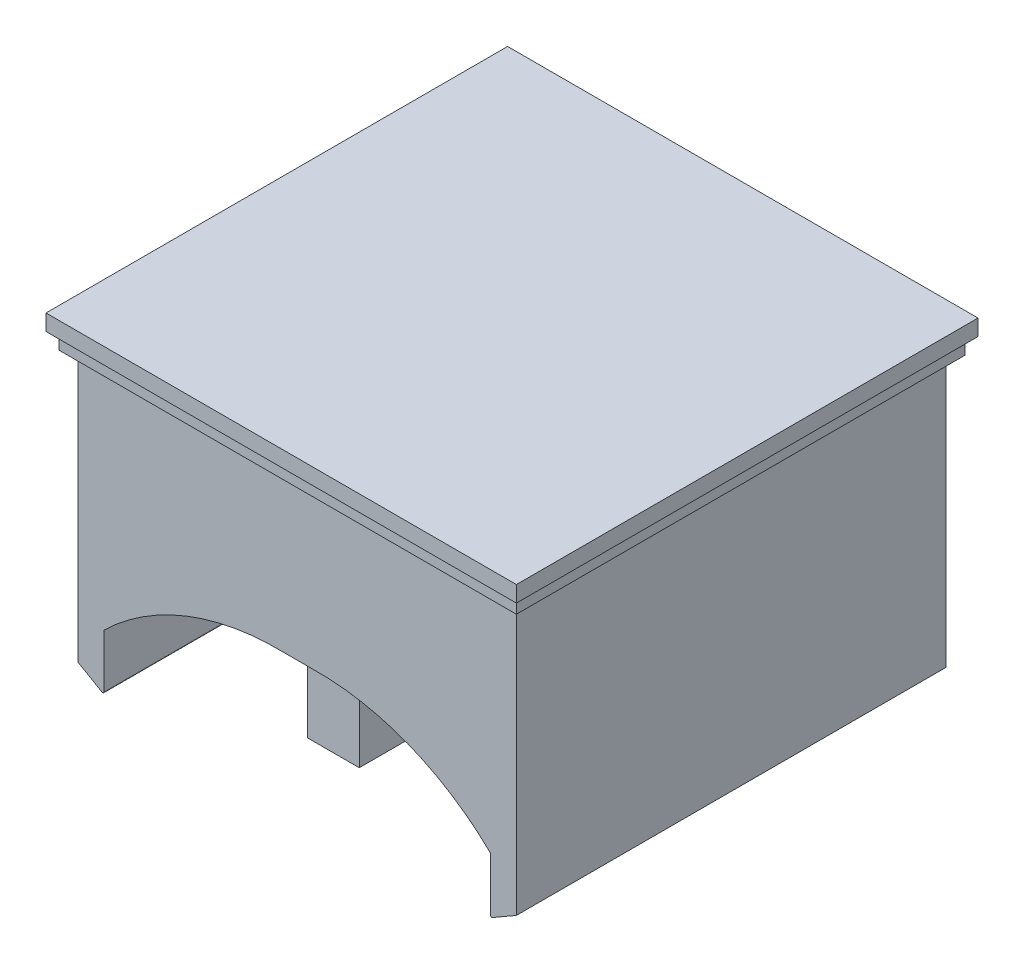
SolidWorks part; units mm, degrees
ref_plane "Front Plane" through (0, 0, 0) normal (0, 0, 1) x (1, 0, 0)
ref_plane "Top Plane" through (0, 0, 0) normal (0, 1, 0) x (1, 0, 0)
ref_plane "Right Plane" through (0, 0, 0) normal (1, 0, 0) x (0, 0, -1)
sketch "Sketch1" plane through (0, 0, 0) normal (0, 0, 1) x (1, 0, 0)
  line L1 (-34.0722, 25.4981) -> (34.0722, 25.4981)
  line L6 (30.3703, -18.6992) -> (34.0722, -16.5619)
  line L7 (30.0253, -10.1731) -> (30.0253, -18.5)
  line L8 (0, 0.77) -> (2.2012, 0.77)
  line L9 (0, 0.77) -> (-2.2012, 0.77)
  line L10 (-30.0253, -10.1731) -> (-30.0253, -18.5)
  line L11 (-30.3703, -18.6992) -> (-34.0722, -16.5619)
  line L12 (-34.0722, -16.5619) -> (-34.0722, 25.4981)
  line L13 (34.0722, -16.5619) -> (34.0722, 25.4981)
  arc A4 (30.3703, -18.6992) -> (30.0253, -18.5) centre (30.2553, -18.5) cw
  arc A5 (2.2012, 0.77) -> (30.0253, -10.1731) centre (3.08, -37.84) cw
  arc A6 (-2.2012, 0.77) -> (-30.0253, -10.1731) centre (-3.08, -37.84) ccw
  arc A7 (-30.3703, -18.6992) -> (-30.0253, -18.5) centre (-30.2553, -18.5) ccw
  dimension "D2" = 1.9381
extrude "Boss-Extrude1" add sketch "Sketch1" against normal blind 66.78
sketch "Sketch3" plane through (0, 25.4981, 0) normal (0, 1, 0) x (1, 0, 0)
  line L4 (-4.03, 61.17) -> (-4.03, 5.61)
  line L5 (-4.03, 5.61) -> (4.03, 5.61)
  line L6 (4.03, 5.61) -> (4.03, 61.17)
  line L7 (4.03, 61.17) -> (-4.03, 61.17)
extrude "Boss-Extrude2" add sketch "Sketch3" against normal blind 40
sketch "Sketch5" plane through (0, 25.4981, 0) normal (0, 1, 0) x (1, 0, 0)
  line L0 (-35.5722, 68.28) -> (35.5722, 68.28)
  line L5 (35.5722, 68.28) -> (35.5722, -1.5)
  line L6 (-35.5722, -1.5) -> (35.5722, -1.5)
  line L7 (-35.5722, 68.28) -> (-35.5722, -1.5)
extrude "Boss-Extrude4" add sketch "Sketch5" along normal blind 2.5
sketch "Sketch6" plane through (0, 27.9981, 0) normal (0, 1, 0) x (1, 0, 0)
  line L0 (-36.5722, 69.28) -> (36.5722, 69.28)
  line L5 (36.5722, 69.28) -> (36.5722, -2.5)
  line L6 (-36.5722, -2.5) -> (36.5722, -2.5)
  line L7 (-36.5722, 69.28) -> (-36.5722, -2.5)
extrude "Boss-Extrude5" add sketch "Sketch6" along normal blind 2.5
sketch "Sketch7" plane through (0, 0, -66.78) normal (0, 0, -1) x (-1, 0, 0)
  line L0 (0, 0.77) -> (0, 19.0954) construction
  circle A0 centre (0, 6.1012) radius 1.5
  circle A1 centre (0, 16.1012) radius 1.5
  dimension "D1" = 10
extrude "Cut-Extrude1" cut sketch "Sketch7" against normal blind 10
